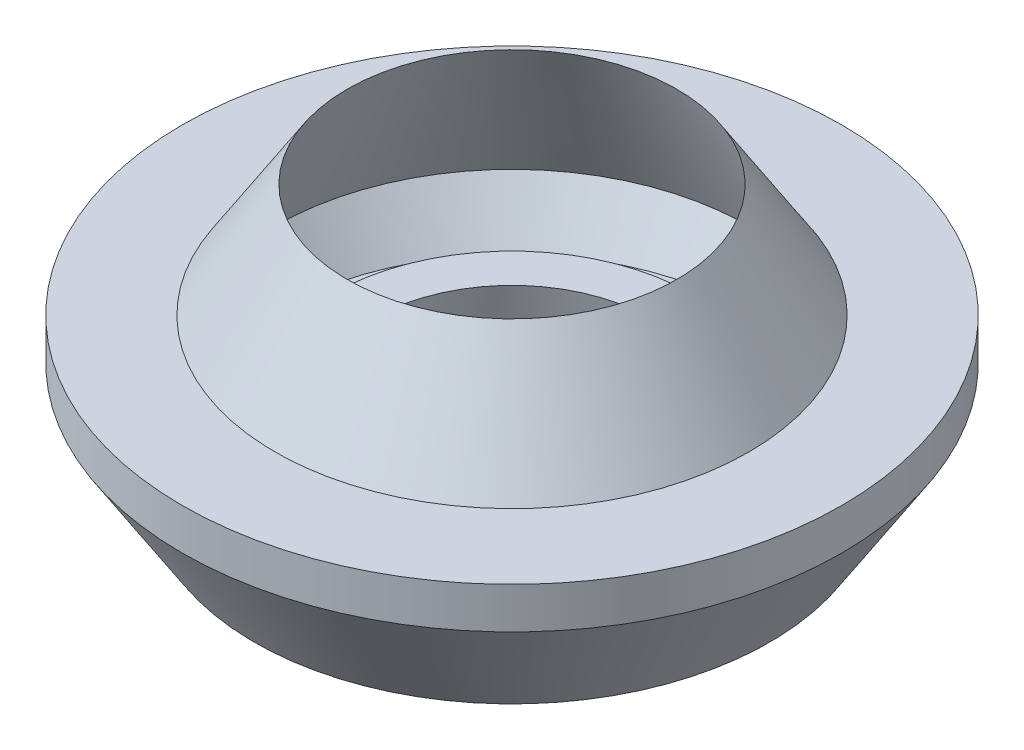
from build123d import *


with BuildPart() as part:
    # Sketch1 → Revolve1 (revolve)
    with BuildSketch(Plane.XY, mode=Mode.PRIVATE) as revolve1_sk:
        Polygon((16, 26), (23, 15), (32, 15), (32, 11), (25, 0), (15, 0), (13.45, 8), (17.524386457, 8), (18.299386457, 4), (22.804216433, 4), (27.258761887, 11), (22.994614872, 11), align=None)
    revolve(revolve1_sk.sketch.rotate(Axis((0, 12.915252942, 0), (0, -1, 0)), 180), axis=Axis((0, 12.915252942, 0), (0, -1, 0)))


solid = part.part
